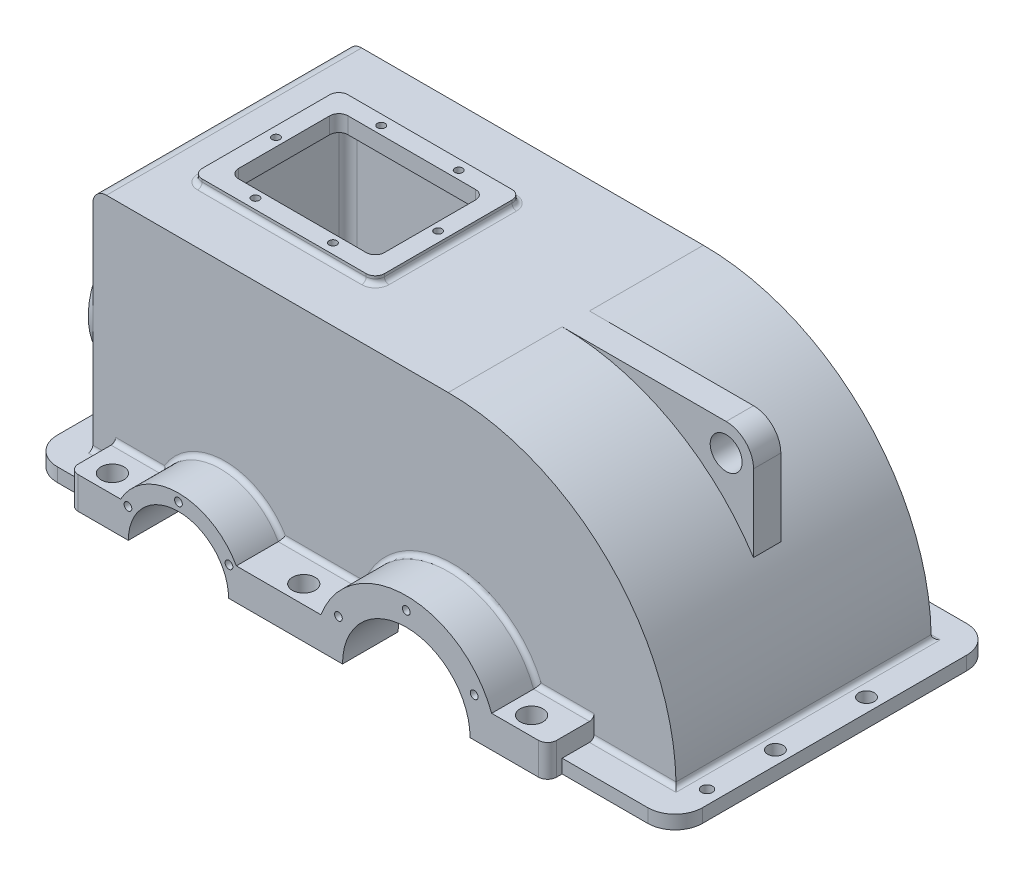
from build123d import *

# Parameters (mm, degrees)
BOSS_EXTRUDE1_DEPTH            = 130
SHELL1_T                       = 10
SKETCH2_W                      = 708
SKETCH2_H                      = 350
BOSS_EXTRUDE2_DEPTH            = 15
FILLET1_R                      = 30
BOSS_EXTRUDE4_DEPTH            = 61
SKETCH8_W                      = 525
SKETCH8_H                      = 61
BOSS_EXTRUDE5_DEPTH            = 35
CUT_EXTRUDE1_REACH             = 692.143
SKETCH9_R                      = 55
SKETCH9_R_2                    = 70
BOSS_EXTRUDE6_DEPTH            = 5
BOSS_EXTRUDE6_DEPTH_BACK       = 53
SKETCH10_R                     = 78
F_1_0_110_DIAMETER_HOLE1_D     = 110
F_1_0_110_DIAMETER_HOLE1_DEPTH = 58
SKETCH21_W                     = 35
SKETCH21_H                     = 134
BOSS_EXTRUDE7_DEPTH            = 185
CUT_EXTRUDE2_REACH             = 495.337
SKETCH22_R                     = 50
SKETCH23_W                     = 2.7
SKETCH23_H                     = 16.25
SKETCH24_R                     = 12.5
CUT_EXTRUDE3_DEPTH             = 580.58778455
SKETCH25_R                     = 8.5
SKETCH25_R_2                   = 6
CUT_EXTRUDE4_DEPTH             = 622.72904066
M10_TAPPED_HOLE9_AT_2_COUNT    = 2
M10_TAPPED_HOLE9_AT_2_PITCH    = 64
M10_TAPPED_HOLE9_AT_3_COUNT    = 2
M10_TAPPED_HOLE9_AT_3_PITCH    = 176.773605601
M10_TAPPED_HOLE9_AT_4_COUNT    = 2
M10_TAPPED_HOLE9_AT_4_PITCH    = 250.966133173
M10_TAPPED_HOLE9_AT_5_COUNT    = 2
M10_TAPPED_HOLE9_AT_5_PITCH    = 325.157027239
SKETCH44_W                     = 160
SKETCH44_H                     = 120
CUT_EXTRUDE6_DEPTH             = 622.72904066
SKETCH46_W                     = 200
SKETCH46_H                     = 160
SKETCH46_W_2                   = 160
SKETCH46_H_2                   = 120
BOSS_EXTRUDE9_DEPTH            = 8
BOSS_EXTRUDE10_DEPTH           = 15
FILLET2_R                      = 30
SKETCH48_R                     = 17.5
CUT_EXTRUDE7_DEPTH             = 624.571166748
CIRPATTERN2_COUNT              = 8
M10_TAPPED_HOLE11_D            = 8.5
FILLET3_R                      = 35
FILLET4_R                      = 15
FILLET5_R                      = 10
FILLET6_R                      = 10
FILLET7_R                      = 10
FILLET8_R                      = 10
FILLET9_R                      = 5
FILLET10_R                     = 5


with BuildPart() as part:
    # Sketch1 → Boss-Extrude1 (new, symmetric)
    with BuildSketch(Plane.XY):
        with BuildLine():
            Line((245, 240), (-135, 240))
            Line((-135, 240), (-135, 0))
            Line((-135, 0), (485, 0))
            ThreePointArc((485, 0), (414.705627485, 169.705627485), (245, 240))
        make_face()
    extrude(amount=BOSS_EXTRUDE1_DEPTH, both=True)

    # Shell1
    shell1_openings = [part.faces().sort_by_distance(p)[0] for p in [
        (175, 0, 0),
    ]]
    offset(amount=SHELL1_T, openings=shell1_openings, kind=Kind.INTERSECTION)

    # Sketch2 → Boss-Extrude2 (add)
    with BuildSketch(Plane.XZ):
        with Locations((175, 0)):
            Rectangle(SKETCH2_W, SKETCH2_H)
        Polygon((485, -130), (245, -130), (-135, -130), (-135, 130), (245, 130), (485, 130), align=None, mode=Mode.SUBTRACT)
    extrude(amount=BOSS_EXTRUDE2_DEPTH)

    # Fillet1
    fillet1_edges = [part.edges().sort_by_distance(p)[0] for p in [
        (529, -7.5, -175),
        (529, -7.5, 175),
        (-179, -7.5, 175),
        (-179, -7.5, -175),
    ]]
    fillet(fillet1_edges, radius=FILLET1_R)

    # Sketch7 → Boss-Extrude4 (add)
    with BuildSketch(Plane(origin=(0, 0, 130), x_dir=(-1, 0, 0), z_dir=(0, 0, -1))):
        with BuildLine():
            ThreePointArc((-150, -15), (-250, 85), (-350, -15))
            Line((-350, -15), (-150, -15))
        make_face()
        with BuildLine():
            ThreePointArc((72.5, -15), (0, 57.5), (-72.5, -15))
            Line((-72.5, -15), (72.5, -15))
        make_face()
    boss_extrude4 = extrude(amount=-BOSS_EXTRUDE4_DEPTH)

    # Sketch8 → Boss-Extrude5 (add)
    with BuildSketch(Plane.XZ.offset(15)):
        with Locations((142.5, 160.5)):
            Rectangle(SKETCH8_W, SKETCH8_H)
    boss_extrude5 = extrude(amount=-BOSS_EXTRUDE5_DEPTH)

    # Sketch9 → Cut-Extrude1 (cut, up to next)
    with BuildSketch(Plane.XY.offset(191), mode=Mode.PRIVATE) as cut_extrude1_sk1:
        with Locations((0, -15)):
            Circle(SKETCH9_R)
    cut_extrude1_tool1 = extrude(cut_extrude1_sk1.sketch, amount=-CUT_EXTRUDE1_REACH, mode=Mode.PRIVATE) & part.part
    # Sketch9 → Cut-Extrude1 (cut, up to next)
    with BuildSketch(Plane.XY.offset(191), mode=Mode.PRIVATE) as cut_extrude1_sk2:
        with Locations((250, -15)):
            Circle(SKETCH9_R_2)
    cut_extrude1_tool2 = extrude(cut_extrude1_sk2.sketch, amount=-CUT_EXTRUDE1_REACH, mode=Mode.PRIVATE) & part.part
    cut_extrude1_1 = cut_extrude1_tool1.solids().sort_by_distance((0, -15, 191))[0]
    add(cut_extrude1_1, mode=Mode.SUBTRACT)
    cut_extrude1_2 = cut_extrude1_tool2.solids().sort_by_distance((250, -15, 191))[0]
    add(cut_extrude1_2, mode=Mode.SUBTRACT)
    cut_extrude1 = cut_extrude1_1 + cut_extrude1_2  # Cut-Extrude1 as one shape, for the pattern or mirror that repeats it

    # Mirror3: Boss-Extrude4, Boss-Extrude5, Cut-Extrude1 across plane
    add(boss_extrude4.mirror(Plane.XY))
    add(boss_extrude5.mirror(Plane.XY))
    add(cut_extrude1.mirror(Plane.XY), mode=Mode.SUBTRACT)

    # Sketch10 → Boss-Extrude6 (add, two sides: drawn at the far end of the back side and taken through both)
    with BuildSketch(Plane.ZY.offset(145).offset(-BOSS_EXTRUDE6_DEPTH_BACK)):
        with Locations(Location((62, 125, 0), (0, 0, 270))):
            Circle(SKETCH10_R)
    extrude(amount=BOSS_EXTRUDE6_DEPTH + BOSS_EXTRUDE6_DEPTH_BACK)

    # Ø1.0 (110) Diameter Hole1
    with Locations(Plane.ZY.offset(150)):
        with Locations((62, 125)):
            Hole(F_1_0_110_DIAMETER_HOLE1_D / 2, depth=F_1_0_110_DIAMETER_HOLE1_DEPTH)

    # Sketch21 → Boss-Extrude7 (add)
    with BuildSketch(Plane.XZ.offset(-240)):
        with Locations((131.5, 63)):
            Rectangle(SKETCH21_W, SKETCH21_H)
    extrude(amount=BOSS_EXTRUDE7_DEPTH)

    # Sketch22 → Cut-Extrude2 (cut, up to next)
    with BuildSketch(Plane(origin=(149, 0, 0), x_dir=(0, 0, -1), z_dir=(1, 0, 0)), mode=Mode.PRIVATE) as cut_extrude2_sk1:
        with Locations((-62, 125)):
            Circle(SKETCH22_R)
    cut_extrude2_tool1 = extrude(cut_extrude2_sk1.sketch, amount=-CUT_EXTRUDE2_REACH, mode=Mode.PRIVATE) & part.part
    add(cut_extrude2_tool1.solids().sort_by_distance((149, 125, 62))[0], mode=Mode.SUBTRACT)

    # Sketch23 → Cut-Revolve1 (revolve, cut)
    with BuildSketch(Plane(origin=(0, 125, 0), x_dir=(-1, 0, 0), z_dir=(0, -1, 0)), mode=Mode.PRIVATE) as cut_revolve1_sk:
        with Locations((-141.6, -105.625)):
            Rectangle(SKETCH23_W, SKETCH23_H)
    revolve(cut_revolve1_sk.sketch.rotate(Axis((-179.001, 125, 62), (1, 0, 0)), 180), axis=Axis((-179.001, 125, 62), (1, 0, 0)), mode=Mode.SUBTRACT)

    # Sketch24 → Cut-Extrude3 (cut, through all)
    with BuildSketch(Plane(origin=(0, 125, 0), x_dir=(-1, 0, 0), z_dir=(0, -1, 0))):
        with Locations(Location((92.5, -171, 0), (0, 0, 90))):
            Circle(SKETCH24_R)
        with Locations(Location((-117.5, -171, 0), (0, 0, 90))):
            Circle(SKETCH24_R)
        with Locations(Location((-367.5, -171, 0), (0, 0, 90))):
            Circle(SKETCH24_R)
    cut_extrude3 = extrude(amount=CUT_EXTRUDE3_DEPTH, mode=Mode.SUBTRACT)

    # Mirror4: Cut-Extrude3 across plane
    add(cut_extrude3.mirror(Plane.XY), mode=Mode.SUBTRACT)

    # Sketch25 → Cut-Extrude4 (cut, through all)
    with BuildSketch(Plane.XZ.offset(15)):
        with Locations((-164, 50)):
            Circle(SKETCH25_R)
        with Locations((-164, -50)):
            Circle(SKETCH25_R)
        with Locations((514, 50)):
            Circle(SKETCH25_R)
        with Locations((514, -50)):
            Circle(SKETCH25_R)
        with Locations((-164, -125)):
            Circle(SKETCH25_R_2)
        with Locations((514, 125)):
            Circle(SKETCH25_R_2)
    extrude(amount=-CUT_EXTRUDE4_DEPTH, mode=Mode.SUBTRACT)

    # Sketch42 → M10 Tapped Hole8 (revolve, cut)
    with BuildSketch(Plane(origin=(-55.425625842, 17, 191), x_dir=(0, -1, 0), z_dir=(1, 0, 0))):
        Polygon((0, 0), (0, 30.053657631), (4.25, 27.5), (4.25, 0), align=None)
    m10_tapped_hole8 = revolve(axis=Axis((-55.425625842, 17, 197.35), (0, 0, -1)), mode=Mode.SUBTRACT)

    # Sketch43 → M10 Tapped Hole9 (revolve, cut)
    with BuildSketch(Plane(origin=(0, 49, 191), x_dir=(0, -1, 0), z_dir=(1, 0, 0))):
        Polygon((0, 0), (0, 30.053657631), (4.25, 27.5), (4.25, 0), align=None)
    m10_tapped_hole9 = revolve(axis=Axis((0, 49, 197.35), (0, 0, -1)), mode=Mode.SUBTRACT)

    # M10 Tapped Hole9 at 2: M10 Tapped Hole9 ×2
    with Locations(*[Vector(0.866025403784438, -0.5000000000000011, 0) * (i * M10_TAPPED_HOLE9_AT_2_PITCH) for i in range(1, M10_TAPPED_HOLE9_AT_2_COUNT)]):
        add(m10_tapped_hole9, mode=Mode.SUBTRACT)

    # M10 Tapped Hole9 at 3: M10 Tapped Hole9 ×2
    with Locations(*[Vector(0.9929186808038332, -0.11879601555092546, 0) * (i * M10_TAPPED_HOLE9_AT_3_PITCH) for i in range(1, M10_TAPPED_HOLE9_AT_3_COUNT)]):
        add(m10_tapped_hole9, mode=Mode.SUBTRACT)

    # M10 Tapped Hole9 at 4: M10 Tapped Hole9 ×2
    with Locations(*[Vector(0.9961503444262931, 0.08766123030951357, 0) * (i * M10_TAPPED_HOLE9_AT_4_PITCH) for i in range(1, M10_TAPPED_HOLE9_AT_4_COUNT)]):
        add(m10_tapped_hole9, mode=Mode.SUBTRACT)

    # M10 Tapped Hole9 at 5: M10 Tapped Hole9 ×2
    with Locations(*[Vector(0.9979122625180912, -0.06458418007549843, 0) * (i * M10_TAPPED_HOLE9_AT_5_PITCH) for i in range(1, M10_TAPPED_HOLE9_AT_5_COUNT)]):
        add(m10_tapped_hole9, mode=Mode.SUBTRACT)

    # Mirror5: M10 Tapped Hole9 across plane
    add(m10_tapped_hole9.mirror(Plane.XY), mode=Mode.SUBTRACT)

    # Mirror5 copy 1 sketch → Mirror5 copy 1 (revolve, cut)
    with BuildSketch(Plane(origin=(55.425625842, 17, -191), x_dir=(0, -1, 0), z_dir=(1, 0, 0))):
        Polygon((0, 0), (0, -30.053657631), (4.25, -27.5), (4.25, 0), align=None)
    revolve(axis=Axis((55.425625842, 17, -197.35), (0, 0, -1)), mode=Mode.SUBTRACT)

    # Mirror5 copy 2 sketch → Mirror5 copy 2 (revolve, cut)
    with BuildSketch(Plane(origin=(175.521815275, 28, -191), x_dir=(0, -1, 0), z_dir=(1, 0, 0))):
        Polygon((0, 0), (0, -30.053657631), (4.25, -27.5), (4.25, 0), align=None)
    revolve(axis=Axis((175.521815275, 28, -197.35), (0, 0, -1)), mode=Mode.SUBTRACT)

    # Mirror5 copy 3 sketch → Mirror5 copy 3 (revolve, cut)
    with BuildSketch(Plane(origin=(250, 71, -191), x_dir=(0, -1, 0), z_dir=(1, 0, 0))):
        Polygon((0, 0), (0, -30.053657631), (4.25, -27.5), (4.25, 0), align=None)
    revolve(axis=Axis((250, 71, -197.35), (0, 0, -1)), mode=Mode.SUBTRACT)

    # Mirror5 copy 4 sketch → Mirror5 copy 4 (revolve, cut)
    with BuildSketch(Plane(origin=(324.478184725, 28, -191), x_dir=(0, -1, 0), z_dir=(1, 0, 0))):
        Polygon((0, 0), (0, -30.053657631), (4.25, -27.5), (4.25, 0), align=None)
    revolve(axis=Axis((324.478184725, 28, -197.35), (0, 0, -1)), mode=Mode.SUBTRACT)

    # Mirror6: M10 Tapped Hole8 across plane
    add(m10_tapped_hole8.mirror(Plane.XY), mode=Mode.SUBTRACT)

    # Sketch44 → Cut-Extrude6 (cut, through all)
    with BuildSketch(Plane(origin=(0, 250, 0), x_dir=(1, 0, 0), z_dir=(0, 1, 0))):
        with Locations((5, 0)):
            Rectangle(SKETCH44_W, SKETCH44_H)
    extrude(amount=-CUT_EXTRUDE6_DEPTH, mode=Mode.SUBTRACT)

    # Sketch46 → Boss-Extrude9 (add)
    with BuildSketch(Plane(origin=(0, 250, 0), x_dir=(1, 0, 0), z_dir=(0, 1, 0))):
        with Locations((5, 0)):
            Rectangle(SKETCH46_W, SKETCH46_H)
        with Locations((5, 0)):
            Rectangle(SKETCH46_W_2, SKETCH46_H_2, mode=Mode.SUBTRACT)
    extrude(amount=BOSS_EXTRUDE9_DEPTH)

    # Sketch47 → Boss-Extrude10 (add, symmetric)
    with BuildSketch(Plane.XY):
        with BuildLine():
            Line((455, 250), (245, 250))
            ThreePointArc((245, 250), (364.558249578, 219.558249578), (455, 135.646599663))
            Line((455, 135.646599663), (455, 250))
        make_face()
    extrude(amount=BOSS_EXTRUDE10_DEPTH, both=True)

    # Fillet2
    fillet2_edges = [part.edges().sort_by_distance(p)[0] for p in [
        (455, 250, 0),
    ]]
    fillet(fillet2_edges, radius=FILLET2_R)

    # Sketch48 → Cut-Extrude7 (cut, through all)
    with BuildSketch(Plane.XY.offset(15)):
        with Locations((425, 220)):
            Circle(SKETCH48_R)
    extrude(amount=-CUT_EXTRUDE7_DEPTH, mode=Mode.SUBTRACT)

    # Sketch50 → M10 Tapped Hole10 (revolve, cut)
    with BuildSketch(Plane(origin=(-150, 192, 62), x_dir=(0, 0, 1), z_dir=(0, 1, 0))):
        Polygon((0, 0), (0, 33.053657631), (4.25, 30.5), (4.25, 0), align=None)
    m10_tapped_hole10 = revolve(axis=Axis((-156.35, 192, 62), (1, 0, 0)), mode=Mode.SUBTRACT)

    # CirPattern2: M10 Tapped Hole10 ×8 about axis
    cirpattern2_axis = Axis((0, 125, 62), (1, 0, 0))
    for i in range(1, CIRPATTERN2_COUNT):
        add(m10_tapped_hole10.rotate(cirpattern2_axis, i * 360 / CIRPATTERN2_COUNT), mode=Mode.SUBTRACT)

    # M10 Tapped Hole11 (through all)
    with Locations(Plane(origin=(0, 258, 0), x_dir=(1, 0, 0), z_dir=(0, 1, 0))):
        with Locations((-37.5, 69), (-84, 0), (94, 0), (47.5, -69), (-37.5, -69), (47.5, 69)):
            Hole(M10_TAPPED_HOLE11_D / 2)

    # Fillet3
    fillet3_edges = [part.edges().sort_by_distance(p)[0] for p in [
        (131.5, 55, -4),
    ]]
    fillet(fillet3_edges, radius=FILLET3_R)

    # Fillet4
    fillet4_edges = [part.edges().sort_by_distance(p)[0] for p in [
        (-145, 250, 0),
    ]]
    fillet(fillet4_edges, radius=FILLET4_R)

    # Fillet5
    fillet5_edges = [part.edges().sort_by_distance(p)[0] for p in [
        (85, 249, -60),
        (85, 249, 60),
        (-75, 249, 60),
        (-75, 249, -60),
        (-95, 254, -80),
        (-95, 254, 80),
        (105, 254, 80),
        (105, 254, -80),
    ]]
    fillet(fillet5_edges, radius=FILLET5_R)

    # Fillet6
    fillet6_edges = [part.edges().sort_by_distance(p)[0] for p in [
        (405, 2.5, 191),
        (-120, 2.5, 191),
    ]]
    fillet(fillet6_edges, radius=FILLET6_R)

    # Fillet7
    fillet7_edges = [part.edges().sort_by_distance(p)[0] for p in [
        (485, -7.5, 130),
        (-135, 35.895026825, 130),
        (-10.5, 240, 130),
        (197, 240, 130),
        (414.705627485, 169.705627485, 130),
        (485, -7.5, -130),
        (-135, 112.5, -130),
        (55, 240, -130),
        (414.705627485, 169.705627485, -130),
        (-135, 240, 0),
    ]]
    fillet(fillet7_edges, radius=FILLET7_R)

    # Fillet8
    fillet8_edges = [part.edges().sort_by_distance(p)[0] for p in [
        (-120, 2.5, -191),
        (405, 2.5, -191),
    ]]
    fillet(fillet8_edges, radius=FILLET8_R)

    # Fillet9
    fillet9_edges = [part.edges().sort_by_distance(p)[0] for p in [
        (5, 250, -80),
        (105, 250, 0),
        (5, 250, 80),
        (-95, 250, 0),
        (102.071067812, 250, -77.071067812),
        (102.071067812, 250, 77.071067812),
        (-92.071067812, 250, 77.071067812),
        (-92.071067812, 250, -77.071067812),
    ]]
    fillet(fillet9_edges, radius=FILLET9_R)

    # Fillet10
    fillet10_edges = [part.edges().sort_by_distance(p)[0] for p in [
        (-132.5, 0, 140),
        (-91.746062748, 20, 140),
        (0, 57.5, 140),
        (109.90857776, 20, 140),
        (250, 85, 140),
        (374.337484988, 20, 140),
        (450, 0, 140),
        (495, 0, 0),
        (450, 0, -140),
        (250, 85, -140),
        (-132.5, 0, -140),
        (-91.746062748, 20, -140),
        (0, 57.5, -140),
        (109.90857776, 20, -140),
    ]]
    fillet(fillet10_edges, radius=FILLET10_R)


solid = part.part
